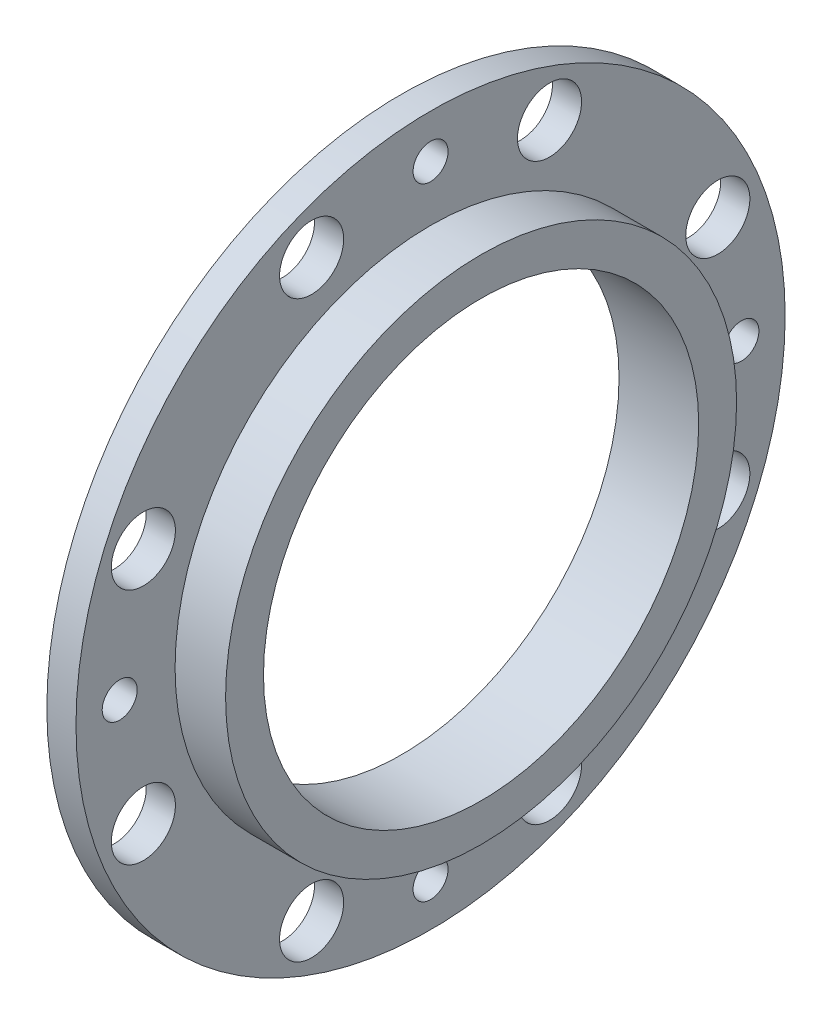
SolidWorks part; units mm, degrees
ref_plane "Front" through (0, 0, 0) normal (0, 0, 1) x (1, 0, 0)
ref_plane "Top" through (0, 0, 0) normal (0, 1, 0) x (1, 0, 0)
ref_plane "Right" through (0, 0, 0) normal (1, 0, 0) x (0, 0, -1)
sketch "Sketch1" plane through (0, 0, 0) normal (0, 0, 1) x (1, 0, 0)
  line L0 (-91.4265, 0) -> (124.6083, 0) construction
  line L1 (-19.589, 112) -> (-19.589, 182.5)
  line L2 (-19.589, 182.5) -> (-4.589, 182.5)
  line L3 (-4.589, 182.5) -> (-4.589, 131.5)
  line L4 (-4.589, 131.5) -> (21.411, 131.5)
  line L5 (21.411, 131.5) -> (21.411, 112)
  line L6 (21.411, 112) -> (-19.589, 112)
  dimension "D1" = 182.5
  dimension "D2" = 15
  dimension "D3" = 41
  dimension "D4" = 131.5
  dimension "D5" = 112
revolve "Revolve1" add sketch "Sketch1" angle 360 about L0
sketch "Sketch2" plane through (-19.589, 0, 0) normal (-1, 0, 0) x (0, 0, 1)
  line L0 (0, 0) -> (0, 198.02) construction
  line L1 (0, 0) -> (69.8397, 168.608) construction
  circle A0 centre (0, 0) radius 160 construction
  circle A1 centre (0, 0) radius 182.5 construction
  circle A2 centre (61.2293, 147.8207) radius 16.5
  circle A3 centre (147.8207, 61.2293) radius 16.5
  circle A4 centre (147.8207, -61.2293) radius 16.5
  circle A5 centre (61.2293, -147.8207) radius 16.5
  circle A6 centre (-61.2293, -147.8207) radius 16.5
  circle A7 centre (-147.8207, -61.2293) radius 16.5
  circle A8 centre (-147.8207, 61.2293) radius 16.5
  circle A9 centre (-61.2293, 147.8207) radius 16.5
  point P25 (0, 0)
  dimension "D1" = 320
  dimension "D3" = 33
  dimension "D2" = 22.5
extrude "Cut-Extrude1" cut sketch "Sketch2" against normal blind 20
sketch "Sketch3" plane through (-19.589, 0, 0) normal (-1, 0, 0) x (0, 0, 1)
  circle A0 centre (0, 0) radius 160 construction
  circle A1 centre (0, 160) radius 9
  circle A2 centre (160, 0) radius 9
  circle A3 centre (0, -160) radius 9
  circle A4 centre (-160, 0) radius 9
  point P14 (0, 0)
  dimension "D1" = 160
extrude "Cut-Extrude2" cut sketch "Sketch3" against normal blind 20
equation "\"零件重量\"= IIF ( \"SW-质量\" > 100 , int ( \"SW-质量\" ) , \"SW-质量\" )"
